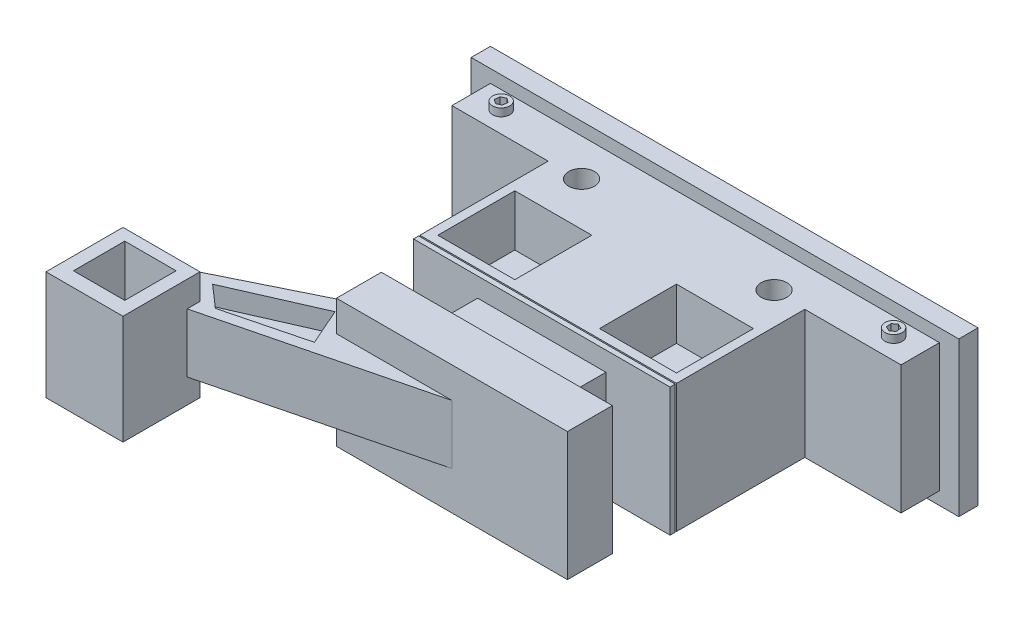
from build123d import *

# Parameters (mm, degrees)
BOSS_EXTRUDE1_DEPTH       = 100
SKETCH2_W                 = 60
SKETCH2_H                 = 60
CUT_EXTRUDE1_DEPTH        = 40
SKETCH3_W                 = 100
SKETCH3_H                 = 40
CUT_EXTRUDE2_DEPTH        = 15
SKETCH4_W                 = 380
SKETCH4_H                 = 120
BOSS_EXTRUDE2_DEPTH       = 15
SKETCH5_R                 = 4
BOSS_EXTRUDE3_DEPTH       = 4
MIRROR4_COPY_1_SKETCH_R   = 4
MIRROR4_COPY_1_DEPTH      = 4
SKETCH6_W                 = 193.699537798
SKETCH6_H                 = 93.725582806
BOSS_EXTRUDE4_DEPTH       = 1
SKETCH7_W                 = 200
SKETCH7_H                 = 100
BOSS_EXTRUDE5_DEPTH       = 4
CUT_EXTRUDE3_REACH        = 345.657
SKETCH8_W                 = 24.755455522
SKETCH8_H                 = 35.4669507
SKETCH9_R                 = 7.5
BOSS_EXTRUDE6_DEPTH       = 1.5
SKETCH10_R                = 5.050087977
BOSS_EXTRUDE7_DEPTH       = 5
MIRROR6_COPY_1_SKETCH_R   = 7.5
MIRROR6_COPY_1_DEPTH      = 1.5
MIRROR6_COPY_2_SKETCH_R   = 5.050087977
MIRROR6_COPY_2_DEPTH      = 5
CUT_EXTRUDE4_REACH        = 374.693
SKETCH11_R                = 10
SKETCH12_R                = 6.712783718
BOSS_EXTRUDE8_DEPTH       = 6
MIRROR8_COPY_1_SKETCH_R   = 6.712783718
MIRROR8_COPY_1_DEPTH      = 6
BOSS_EXTRUDE9_DEPTH       = 26
BOSS_EXTRUDE9_DEPTH_BACK  = 20
SKETCH13_W                = 40
SKETCH13_H                = 40
BOSS_EXTRUDE10_DEPTH      = 20
BOSS_EXTRUDE10_DEPTH_BACK = 65
SKETCH14_W                = 60
SKETCH14_H                = 60
SKETCH14_W_2              = 40
SKETCH14_H_2              = 40
CUT_EXTRUDE5_DEPTH        = 15


with BuildPart() as part:
    # Sketch1 → Boss-Extrude1 (new body)
    with BuildSketch(Plane(origin=(0, 0, 0), x_dir=(1, 0, 0), z_dir=(0, 1, 0))):
        Polygon((0, 0), (0, 35), (40, 35), (40, 75), (-10, 75), (-10, 175), (-85, 175), (-85, 220), (265, 220), (265, 175), (190, 175), (190, 75), (140, 75), (140, 35), (180, 35), (180, 0), align=None)
    extrude(amount=BOSS_EXTRUDE1_DEPTH)

    # Sketch2 → Cut-Extrude1 (cut)
    with BuildSketch(Plane(origin=(0, 100, 0), x_dir=(1, 0, 0), z_dir=(0, 1, 0))):
        with Locations((27, 112)):
            Rectangle(SKETCH2_W, SKETCH2_H)
        with Locations((153, 112)):
            Rectangle(SKETCH2_W, SKETCH2_H)
    cut_extrude1 = extrude(amount=-CUT_EXTRUDE1_DEPTH, mode=Mode.SUBTRACT)

    # Mirror1: Cut-Extrude1 across plane
    add(cut_extrude1.mirror(Plane.ZX.offset(50)), mode=Mode.SUBTRACT)

    # Sketch3 → Cut-Extrude2 (cut)
    with BuildSketch(Plane(origin=(0, 100, 0), x_dir=(1, 0, 0), z_dir=(0, 1, 0))):
        with Locations((90, 55)):
            Rectangle(SKETCH3_W, SKETCH3_H)
    cut_extrude2 = extrude(amount=-CUT_EXTRUDE2_DEPTH, mode=Mode.SUBTRACT)

    # Mirror2: Cut-Extrude2 across plane
    add(cut_extrude2.mirror(Plane.ZX.offset(50)), mode=Mode.SUBTRACT)

    # Sketch4 → Boss-Extrude2 (add)
    with BuildSketch(Plane(origin=(0, 0, -220), x_dir=(-1, 0, 0), z_dir=(0, 0, -1))):
        with Locations((-90, 50)):
            Rectangle(SKETCH4_W, SKETCH4_H)
    extrude(amount=-BOSS_EXTRUDE2_DEPTH)

    # Sketch5 → Boss-Extrude3 (add)
    with BuildSketch(Plane(origin=(0, 0, -82), x_dir=(-1, 0, 0), z_dir=(0, 0, -1))):
        with Locations((-9, 12)):
            Circle(SKETCH5_R)
        Polygon((-7.384647212, 10.364354029), (-6.775812643, 12.581113565), (-8.391165431, 14.216759536), (-10.615352788, 13.635645971), (-11.224187357, 11.418886435), (-9.608834569, 9.783240464), align=None, mode=Mode.SUBTRACT)
    boss_extrude3 = extrude(amount=BOSS_EXTRUDE3_DEPTH)

    # Mirror3: Boss-Extrude3 across plane
    add(boss_extrude3.mirror(Plane.ZY.offset(-90)))

    # Mirror4: Boss-Extrude3 across plane
    add(boss_extrude3.mirror(Plane.ZX.offset(50)))

    # Mirror4 copy 1 sketch → Mirror4 copy 1 (add)
    with BuildSketch(Plane(origin=(180, 100, -82), x_dir=(1, 0, 0), z_dir=(0, 0, -1))):
        with Locations((-9, 12)):
            Circle(MIRROR4_COPY_1_SKETCH_R)
        Polygon((-7.384647212, 10.364354029), (-6.775812643, 12.581113565), (-8.391165431, 14.216759536), (-10.615352788, 13.635645971), (-11.224187357, 11.418886435), (-9.608834569, 9.783240464), align=None, mode=Mode.SUBTRACT)
    extrude(amount=MIRROR4_COPY_1_DEPTH)

    # Sketch6 → Boss-Extrude4 (add)
    with BuildSketch(Plane.XY.offset(-75)):
        with Locations((90, 50)):
            Rectangle(SKETCH6_W, SKETCH6_H)
    extrude(amount=BOSS_EXTRUDE4_DEPTH)

    # Sketch7 → Boss-Extrude5 (add)
    with BuildSketch(Plane.XY.offset(-74)):
        with Locations((90, 50)):
            Rectangle(SKETCH7_W, SKETCH7_H)
    extrude(amount=BOSS_EXTRUDE5_DEPTH)

    # Sketch8 → Cut-Extrude3 (cut, up to next)
    with BuildSketch(Plane(origin=(140, 0, 0), x_dir=(0, 0, -1), z_dir=(1, 0, 0)), mode=Mode.PRIVATE) as cut_extrude3_sk1:
        with Locations((52.991042332, 49.761966774)):
            Rectangle(SKETCH8_W, SKETCH8_H)
    cut_extrude3_tool1 = extrude(cut_extrude3_sk1.sketch, amount=-CUT_EXTRUDE3_REACH, mode=Mode.PRIVATE) & part.part
    add(cut_extrude3_tool1.solids().sort_by_distance((140, 49.761967, -52.991042))[0], mode=Mode.SUBTRACT)

    # Sketch9 → Boss-Extrude6 (add)
    with BuildSketch(Plane(origin=(0, 0, -35), x_dir=(-1, 0, 0), z_dir=(0, 0, -1))):
        with Locations(Location((-168, 88, 0), (0, 0, 180))):
            Circle(SKETCH9_R)
    boss_extrude6 = extrude(amount=BOSS_EXTRUDE6_DEPTH)

    # Sketch10 → Boss-Extrude7 (add)
    with BuildSketch(Plane(origin=(0, 0, -36.5), x_dir=(-1, 0, 0), z_dir=(0, 0, -1))):
        with Locations((-168, 88)):
            Circle(SKETCH10_R)
        Polygon((-169.083119514, 85.45890515), (-166.340907063, 85.791443561), (-165.25778755, 88.332538411), (-166.916880486, 90.54109485), (-169.659092937, 90.208556439), (-170.74221245, 87.667461589), align=None, mode=Mode.SUBTRACT)
    boss_extrude7 = extrude(amount=BOSS_EXTRUDE7_DEPTH)

    # Mirror5: Boss-Extrude6, Boss-Extrude7 across plane
    add(boss_extrude6.mirror(Plane.ZY.offset(-90)))
    add(boss_extrude7.mirror(Plane.ZY.offset(-90)))

    # Mirror6: Boss-Extrude6, Boss-Extrude7 across plane
    add(boss_extrude6.mirror(Plane.ZX.offset(50)))
    add(boss_extrude7.mirror(Plane.ZX.offset(50)))

    # Mirror6 copy 1 sketch → Mirror6 copy 1 (add)
    with BuildSketch(Plane(origin=(180, 100, -35), x_dir=(1, 0, 0), z_dir=(0, 0, -1))):
        with Locations(Location((-168, 88, 0), (0, 0, 180))):
            Circle(MIRROR6_COPY_1_SKETCH_R)
    extrude(amount=MIRROR6_COPY_1_DEPTH)

    # Mirror6 copy 2 sketch → Mirror6 copy 2 (add)
    with BuildSketch(Plane(origin=(180, 100, -36.5), x_dir=(1, 0, 0), z_dir=(0, 0, -1))):
        with Locations((-168, 88)):
            Circle(MIRROR6_COPY_2_SKETCH_R)
        Polygon((-169.083119514, 85.45890515), (-166.340907063, 85.791443561), (-165.25778755, 88.332538411), (-166.916880486, 90.54109485), (-169.659092937, 90.208556439), (-170.74221245, 87.667461589), align=None, mode=Mode.SUBTRACT)
    extrude(amount=MIRROR6_COPY_2_DEPTH)

    # Sketch11 → Cut-Extrude4 (cut, up to next)
    with BuildSketch(Plane(origin=(0, 100, 0), x_dir=(1, 0, 0), z_dir=(0, 1, 0)), mode=Mode.PRIVATE) as cut_extrude4_sk1:
        with Locations(Location((15, 176.040744125, 0), (0, 0, 270))):
            Circle(SKETCH11_R)
    cut_extrude4_tool1 = extrude(cut_extrude4_sk1.sketch, amount=-CUT_EXTRUDE4_REACH, mode=Mode.PRIVATE) & part.part
    # Sketch11 → Cut-Extrude4 (cut, up to next)
    with BuildSketch(Plane(origin=(0, 100, 0), x_dir=(1, 0, 0), z_dir=(0, 1, 0)), mode=Mode.PRIVATE) as cut_extrude4_sk2:
        with Locations(Location((165, 176.040744125, 0), (0, 0, 270))):
            Circle(SKETCH11_R)
    cut_extrude4_tool2 = extrude(cut_extrude4_sk2.sketch, amount=-CUT_EXTRUDE4_REACH, mode=Mode.PRIVATE) & part.part
    add(cut_extrude4_tool1.solids().sort_by_distance((15, 100, -176.040744))[0], mode=Mode.SUBTRACT)
    add(cut_extrude4_tool2.solids().sort_by_distance((165, 100, -176.040744))[0], mode=Mode.SUBTRACT)

    # Sketch12 → Boss-Extrude8 (add)
    with BuildSketch(Plane(origin=(0, 100, 0), x_dir=(1, 0, 0), z_dir=(0, 1, 0))):
        with Locations(Location((-62.933741196, 191.326238388, 0), (0, 0, 90))):
            Circle(SKETCH12_R)
        Polygon((-59.648884866, 188.96276102), (-59.244481589, 192.989268734), (-62.52933792, 195.352746102), (-66.218597527, 193.689715756), (-66.623000804, 189.663208042), (-63.338144473, 187.299730674), align=None, mode=Mode.SUBTRACT)
    boss_extrude8 = extrude(amount=BOSS_EXTRUDE8_DEPTH)

    # Mirror7: Boss-Extrude8 across plane
    add(boss_extrude8.mirror(Plane.ZY.offset(-90)))

    # Mirror8: Boss-Extrude8 across plane
    add(boss_extrude8.mirror(Plane.ZX.offset(50)))

    # Mirror8 copy 1 sketch → Mirror8 copy 1 (add)
    with BuildSketch(Plane(origin=(180, 0, 0), x_dir=(-1, 0, 0), z_dir=(0, -1, 0))):
        with Locations(Location((-62.933741196, 191.326238388, 0), (0, 0, 90))):
            Circle(MIRROR8_COPY_1_SKETCH_R)
        Polygon((-59.648884866, 188.96276102), (-59.244481589, 192.989268734), (-62.52933792, 195.352746102), (-66.218597527, 193.689715756), (-66.623000804, 189.663208042), (-63.338144473, 187.299730674), align=None, mode=Mode.SUBTRACT)
    extrude(amount=MIRROR8_COPY_1_DEPTH)

    # Sketch13 → Boss-Extrude9 (add, two sides: drawn at the far end of the back side and taken through both)
    with BuildSketch(Plane(origin=(0, 50, 0), x_dir=(1, 0, 0), z_dir=(0, 1, 0)).offset(-BOSS_EXTRUDE9_DEPTH_BACK)):
        Polygon((-135, -31.383702087), (-135, -91.383702087), (-75, -91.383702087), (-75, -41.383702087), (90, 0), (0, 35), align=None)
        with Locations((-105, -60)):
            Rectangle(SKETCH13_W, SKETCH13_H, mode=Mode.SUBTRACT)
    extrude(amount=BOSS_EXTRUDE9_DEPTH + BOSS_EXTRUDE9_DEPTH_BACK)

    # Sketch14 → Boss-Extrude10 (add, two sides: drawn at the far end of the back side and taken through both)
    with BuildSketch(Plane(origin=(0, 76, 0), x_dir=(1, 0, 0), z_dir=(0, 1, 0)).offset(-BOSS_EXTRUDE10_DEPTH_BACK)):
        with Locations((-105, -61.383702087)):
            Rectangle(SKETCH14_W, SKETCH14_H)
        with Locations((-105, -60)):
            Rectangle(SKETCH14_W_2, SKETCH14_H_2, mode=Mode.SUBTRACT)
    extrude(amount=BOSS_EXTRUDE10_DEPTH + BOSS_EXTRUDE10_DEPTH_BACK)

    # Sketch15 → Cut-Extrude5 (cut)
    with BuildSketch(Plane(origin=(0, 76, 0), x_dir=(1, 0, 0), z_dir=(0, 1, 0))):
        Polygon((-81.724024622, -14.810070192), (-15.435694668, 14.31332723), (-2.82993923, -14.378877311), (-64.323042641, -30.065725628), align=None)
    cut_extrude5 = extrude(amount=-CUT_EXTRUDE5_DEPTH, mode=Mode.SUBTRACT)

    # Mirror11: Cut-Extrude5 across plane
    add(cut_extrude5.mirror(Plane.ZX.offset(50)), mode=Mode.SUBTRACT)


solid = part.part
